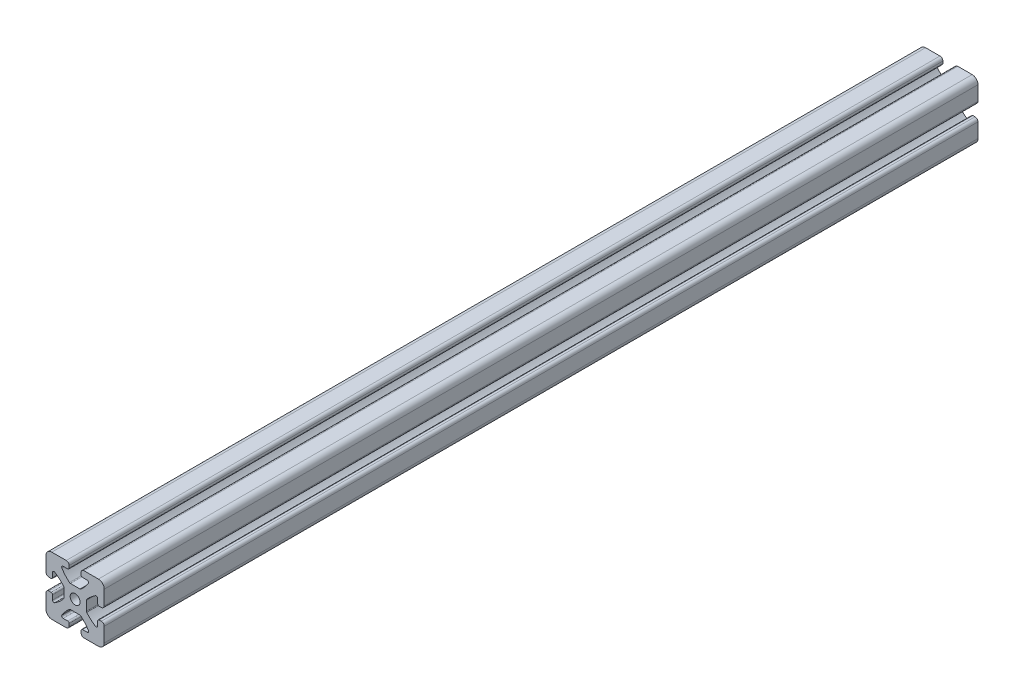
from build123d import *

# Parameters (mm, degrees)
SKETCH1_R           = 3.4
BOSS_EXTRUDE1_DEPTH = 600


with BuildPart() as part:
    # Sketch1 → Boss-Extrude1 (new body)
    with BuildSketch(Plane.XY):
        with BuildLine():
            Line((-72.552625451, -20.1458069), (-75.708839475, -20.1458069))
            ThreePointArc((-75.708839475, -20.1458069), (-76.585125865, -19.62759748), (-76.55321253, -18.610051226))
            ThreePointArc((-76.55321253, -18.610051226), (-74.186362214, -15.403020453), (-71.332517782, -12.620467892))
            ThreePointArc((-71.332517782, -12.620467892), (-71.036129936, -12.453644757), (-70.700972516, -12.3958069))
            Line((-70.700972516, -12.3958069), (-67.452625451, -12.3958069))
            Line((-67.452625451, -12.3958069), (-64.204278386, -12.3958069))
            ThreePointArc((-64.204278386, -12.3958069), (-63.869120967, -12.453644757), (-63.572733121, -12.620467892))
            ThreePointArc((-63.572733121, -12.620467892), (-60.718888688, -15.403020453), (-58.352038372, -18.610051226))
            ThreePointArc((-58.352038372, -18.610051226), (-58.320125037, -19.62759748), (-59.196411427, -20.1458069))
            Line((-59.196411427, -20.1458069), (-62.352625451, -20.1458069))
            ThreePointArc((-62.352625451, -20.1458069), (-63.059732232, -20.438700119), (-63.352625451, -21.1458069))
            Line((-63.352625451, -21.1458069), (-63.352625451, -22.6458069))
            ThreePointArc((-63.352625451, -22.6458069), (-62.766839013, -24.060020463), (-61.352625451, -24.6458069))
            Line((-61.352625451, -24.6458069), (-51.452625451, -24.6458069))
            ThreePointArc((-51.452625451, -24.6458069), (-48.624198326, -23.474234025), (-47.452625451, -20.6458069))
            Line((-47.452625451, -20.6458069), (-47.452625451, -10.7458069))
            ThreePointArc((-47.452625451, -10.7458069), (-48.038411889, -9.331593338), (-49.452625451, -8.7458069))
            Line((-49.452625451, -8.7458069), (-50.952625451, -8.7458069))
            ThreePointArc((-50.952625451, -8.7458069), (-51.659732232, -9.038700119), (-51.952625451, -9.7458069))
            Line((-51.952625451, -9.7458069), (-51.952625451, -12.902020924))
            ThreePointArc((-51.952625451, -12.902020924), (-52.470834871, -13.778307314), (-53.488381126, -13.74639398))
            ThreePointArc((-53.488381126, -13.74639398), (-56.695411898, -11.379543663), (-59.477964459, -8.525699231))
            ThreePointArc((-59.477964459, -8.525699231), (-59.644787594, -8.229311385), (-59.702625451, -7.894153965))
            Line((-59.702625451, -7.894153965), (-59.702625451, -4.6458069))
            Line((-59.702625451, -4.6458069), (-59.702625451, -1.397459836))
            ThreePointArc((-59.702625451, -1.397459836), (-59.644787594, -1.062302416), (-59.477964459, -0.76591457))
            ThreePointArc((-59.477964459, -0.76591457), (-56.695411898, 2.087929862), (-53.488381126, 4.454780179))
            ThreePointArc((-53.488381126, 4.454780179), (-52.470834871, 4.486693513), (-51.952625451, 3.610407123))
            Line((-51.952625451, 3.610407123), (-51.952625451, 0.4541931))
            ThreePointArc((-51.952625451, 0.4541931), (-51.659732232, -0.252913682), (-50.952625451, -0.5458069))
            Line((-50.952625451, -0.5458069), (-49.452625451, -0.5458069))
            ThreePointArc((-49.452625451, -0.5458069), (-48.038411889, 0.039979537), (-47.452625451, 1.4541931))
            Line((-47.452625451, 1.4541931), (-47.452625451, 11.3541931))
            ThreePointArc((-47.452625451, 11.3541931), (-48.624198326, 14.182620224), (-51.452625451, 15.3541931))
            Line((-51.452625451, 15.3541931), (-61.352625451, 15.3541931))
            ThreePointArc((-61.352625451, 15.3541931), (-62.766839013, 14.768406662), (-63.352625451, 13.3541931))
            Line((-63.352625451, 13.3541931), (-63.352625451, 11.8541931))
            ThreePointArc((-63.352625451, 11.8541931), (-63.059732232, 11.147086318), (-62.352625451, 10.8541931))
            Line((-62.352625451, 10.8541931), (-59.196411427, 10.8541931))
            ThreePointArc((-59.196411427, 10.8541931), (-58.320125037, 10.335983679), (-58.352038372, 9.318437425))
            ThreePointArc((-58.352038372, 9.318437425), (-60.718888688, 6.111406652), (-63.572733121, 3.328854091))
            ThreePointArc((-63.572733121, 3.328854091), (-63.869120967, 3.162030956), (-64.204278386, 3.1041931))
            Line((-64.204278386, 3.1041931), (-67.452625451, 3.1041931))
            Line((-67.452625451, 3.1041931), (-70.700972516, 3.1041931))
            ThreePointArc((-70.700972516, 3.1041931), (-71.036129936, 3.162030956), (-71.332517782, 3.328854091))
            ThreePointArc((-71.332517782, 3.328854091), (-74.186362214, 6.111406652), (-76.55321253, 9.318437425))
            ThreePointArc((-76.55321253, 9.318437425), (-76.585125865, 10.335983679), (-75.708839475, 10.8541931))
            Line((-75.708839475, 10.8541931), (-72.552625451, 10.8541931))
            ThreePointArc((-72.552625451, 10.8541931), (-71.84551867, 11.147086318), (-71.552625451, 11.8541931))
            Line((-71.552625451, 11.8541931), (-71.552625451, 13.3541931))
            ThreePointArc((-71.552625451, 13.3541931), (-72.138411889, 14.768406662), (-73.552625451, 15.3541931))
            Line((-73.552625451, 15.3541931), (-83.452625451, 15.3541931))
            ThreePointArc((-83.452625451, 15.3541931), (-86.281052576, 14.182620224), (-87.452625451, 11.3541931))
            Line((-87.452625451, 11.3541931), (-87.452625451, 1.4541931))
            ThreePointArc((-87.452625451, 1.4541931), (-86.866839013, 0.039979537), (-85.452625451, -0.5458069))
            Line((-85.452625451, -0.5458069), (-83.952625451, -0.5458069))
            ThreePointArc((-83.952625451, -0.5458069), (-83.24551867, -0.252913682), (-82.952625451, 0.4541931))
            Line((-82.952625451, 0.4541931), (-82.952625451, 3.610407123))
            ThreePointArc((-82.952625451, 3.610407123), (-82.434416031, 4.486693513), (-81.416869776, 4.454780179))
            ThreePointArc((-81.416869776, 4.454780179), (-78.209839004, 2.087929862), (-75.427286443, -0.76591457))
            ThreePointArc((-75.427286443, -0.76591457), (-75.260463308, -1.062302416), (-75.202625451, -1.397459836))
            Line((-75.202625451, -1.397459836), (-75.202625451, -4.6458069))
            Line((-75.202625451, -4.6458069), (-75.202625451, -7.894153965))
            ThreePointArc((-75.202625451, -7.894153965), (-75.260463308, -8.229311385), (-75.427286443, -8.525699231))
            ThreePointArc((-75.427286443, -8.525699231), (-78.209839004, -11.379543663), (-81.416869776, -13.74639398))
            ThreePointArc((-81.416869776, -13.74639398), (-82.434416031, -13.778307314), (-82.952625451, -12.902020924))
            Line((-82.952625451, -12.902020924), (-82.952625451, -9.7458069))
            ThreePointArc((-82.952625451, -9.7458069), (-83.24551867, -9.038700119), (-83.952625451, -8.7458069))
            Line((-83.952625451, -8.7458069), (-85.452625451, -8.7458069))
            ThreePointArc((-85.452625451, -8.7458069), (-86.866839013, -9.331593338), (-87.452625451, -10.7458069))
            Line((-87.452625451, -10.7458069), (-87.452625451, -20.6458069))
            ThreePointArc((-87.452625451, -20.6458069), (-86.281052576, -23.474234025), (-83.452625451, -24.6458069))
            Line((-83.452625451, -24.6458069), (-73.552625451, -24.6458069))
            ThreePointArc((-73.552625451, -24.6458069), (-72.138411889, -24.060020463), (-71.552625451, -22.6458069))
            Line((-71.552625451, -22.6458069), (-71.552625451, -21.1458069))
            ThreePointArc((-71.552625451, -21.1458069), (-71.84551867, -20.438700119), (-72.552625451, -20.1458069))
        make_face()
        with Locations((-67.452625451, -4.6458069)):
            Circle(SKETCH1_R, mode=Mode.SUBTRACT)
    extrude(amount=BOSS_EXTRUDE1_DEPTH)


solid = part.part
